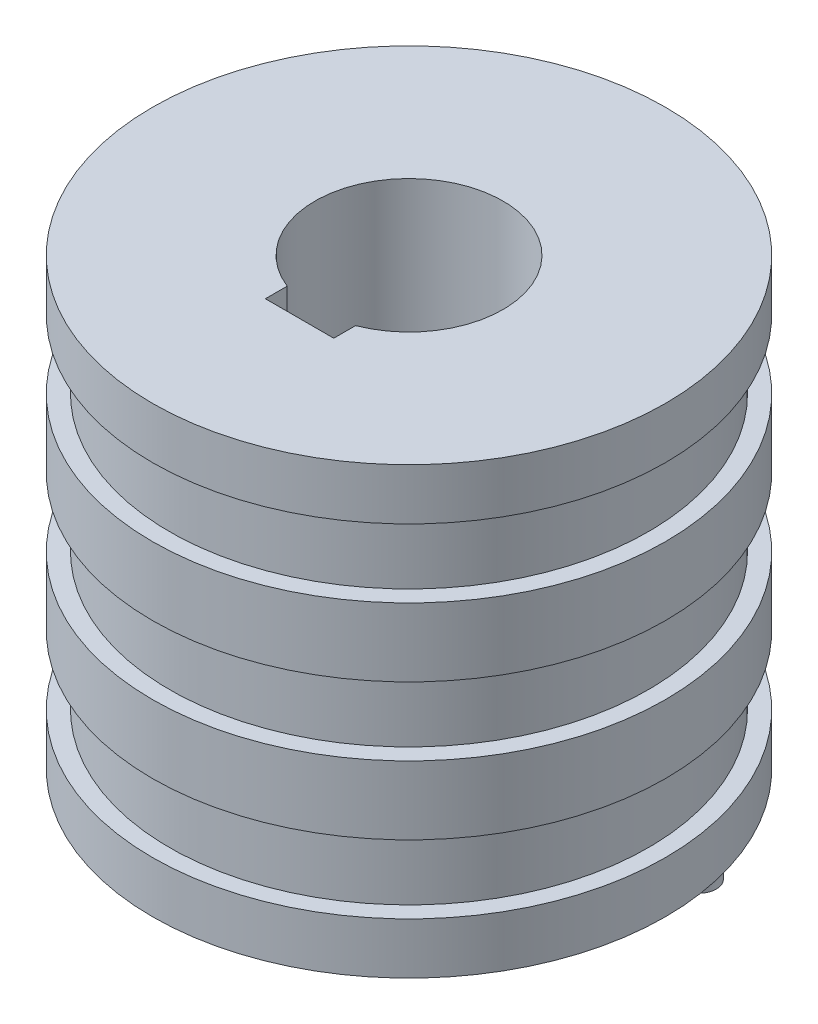
SolidWorks part; units mm, degrees
material "Q235B"
ref_plane "Front Plane" through (0, 0, 0) normal (0, 0, 1) x (1, 0, 0)
ref_plane "Top Plane" through (0, 0, 0) normal (0, 1, 0) x (1, 0, 0)
ref_plane "Right Plane" through (0, 0, 0) normal (1, 0, 0) x (0, 0, -1)
sketch "Sketch 1" plane through (0, 0, 0) normal (0, 0, 1) x (1, 0, 0)
  line L0 (75, 75) -> (70, 75)
  line L1 (0, 0) -> (75, 0)
  line L2 (0, 0) -> (0, 130)
  line L3 (0, 130) -> (75, 130)
  line L4 (75, 0) -> (75, 130)
  line L5 (75, 35) -> (70, 35)
  line L6 (75, 35) -> (75, 15)
  line L7 (75, 15) -> (70, 15)
  line L8 (70, 35) -> (70, 15)
  line L9 (70, 75) -> (70, 55)
  line L10 (75, 55) -> (70, 55)
  line L11 (75, 115) -> (70, 115)
  line L12 (70, 115) -> (70, 95)
  line L13 (75, 95) -> (70, 95)
  line L14 (75, 130) -> (75, 0)
  dimension "D1" = 75
  dimension "D2" = 130
  dimension "D3" = 15
  dimension "D4" = 5
  dimension "D5" = 20
  dimension "D6" = 3
revolve "Revolve1" add sketch "Sketch 1" angle 360 about L2
sketch "Sketch3" plane through (0, 130, 0) normal (0, 1, 0) x (1, 0, 0)
  line L1 (-10, -32) -> (10, -32)
  line L2 (-10, -32) -> (-10, -23)
  line L3 (-10, -23) -> (10, -23)
  line L4 (10, -32) -> (10, -23)
  line L5 (-10, -32) -> (10, -23) construction
  line L6 (-10, -23) -> (10, -32) construction
  circle A0 centre (0, 0) radius 27.5
  point P3 (0, -27.5)
  dimension "D1" = 55
  dimension "D2" = 32
  dimension "D3" = 20
extrude "Cut-Extrude1" cut sketch "Sketch3" against normal blind 130 contours A0 | L1 L4 L3 L2
sketch "Sketch4" plane through (0, 0, 0) normal (0, -1, 0) x (1, 0, 0)
  line L0 (0, 0) -> (46.4783, 0)
  circle A3 centre (0, -60) radius 5
  circle A4 centre (42.425, -42.4278) radius 5
  circle A5 centre (-42.425, -42.4278) radius 5
  dimension "D9" = 10
  dimension "D10" = 10
  dimension "D11" = 10
  dimension "D12" = 84.85
  dimension "D13" = 42.425
  dimension "D14" = 60
  dimension "D15" = 60
  dimension "D16" = 60
extrude "Boss-Extrude3" add sketch "Sketch4" along normal blind 28 contours A5 | A3 | A4
